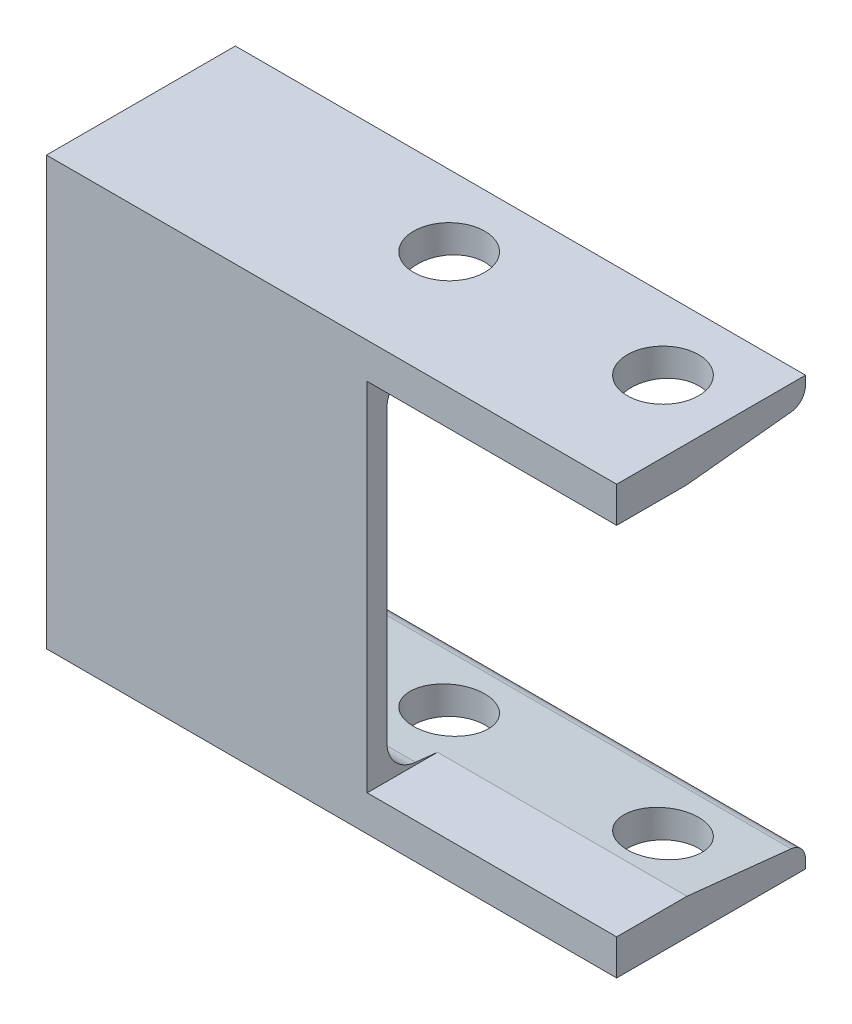
from build123d import *

# Parameters (mm, degrees)
MEMBER_C_12_1_DEPTH = 160
SKETCH_2_W          = 100
SKETCH_2_H          = 100
CUT_EXTRUDE_1_DEPTH = 40
CUT_EXTRUDE_2_REACH = 208.903
SKETCH_3_R          = 10


with BuildPart() as part:
    # Sketch11 → Member C _ 12_1 (new body)
    with BuildSketch(Plane(origin=(0, 0, 0), x_dir=(0, 0, -1), z_dir=(1, 0, 0))):
        with BuildLine():
            Line((53, 120), (0, 120))
            Line((0, 120), (0, 0))
            Line((0, 0), (53, 0))
            Line((53, 0), (53, 2.451956213))
            ThreePointArc((53, 2.451956213), (51.844151715, 5.463043942), (48.970378085, 6.927304742))
            Line((48.970378085, 6.927304742), (13.559243831, 10.649164928))
            ThreePointArc((13.559243831, 10.649164928), (7.811696571, 13.577686529), (5.5, 19.599861986))
            Line((5.5, 19.599861986), (5.5, 100.400138014))
            ThreePointArc((5.5, 100.400138014), (7.811696571, 106.422313471), (13.559243831, 109.350835072))
            Line((13.559243831, 109.350835072), (48.970378085, 113.072695258))
            ThreePointArc((48.970378085, 113.072695258), (51.844151715, 114.536956058), (53, 117.548043787))
            Line((53, 117.548043787), (53, 120))
        make_face()
    extrude(amount=MEMBER_C_12_1_DEPTH)

    # 草图2 → 切除-拉伸1 (cut)
    with BuildSketch(Plane.XY):
        with Locations((140, 60)):
            Rectangle(SKETCH_2_W, SKETCH_2_H)
    extrude(amount=-CUT_EXTRUDE_1_DEPTH, mode=Mode.SUBTRACT)

    # 切除-拉伸2: up to this face of the body (flat: up to its plane)
    cut_extrude_2_end = Plane(part.part.faces().sort_by_distance((80, 120, -26.5))[0])
    # 草图3 → 切除-拉伸2 (cut, up to the picked face)
    with BuildSketch(Plane.XZ, mode=Mode.PRIVATE) as cut_extrude_2_sk1:
        with Locations(Location((140, -33, 0), (0, 0, 270))):
            Circle(SKETCH_3_R)
    cut_extrude_2_tool1 = split(extrude(cut_extrude_2_sk1.sketch, amount=-CUT_EXTRUDE_2_REACH, mode=Mode.PRIVATE), bisect_by=cut_extrude_2_end, keep=Keep.BOTH, mode=Mode.PRIVATE)
    # 草图3 → 切除-拉伸2 (cut, up to the picked face)
    with BuildSketch(Plane.XZ, mode=Mode.PRIVATE) as cut_extrude_2_sk2:
        with Locations(Location((80, -33, 0), (0, 0, 270))):
            Circle(SKETCH_3_R)
    cut_extrude_2_tool2 = split(extrude(cut_extrude_2_sk2.sketch, amount=-CUT_EXTRUDE_2_REACH, mode=Mode.PRIVATE), bisect_by=cut_extrude_2_end, keep=Keep.BOTH, mode=Mode.PRIVATE)
    add(cut_extrude_2_tool1.solids().sort_by(Axis((140, 0, -33), (0, 1, 0)))[0], mode=Mode.SUBTRACT)
    add(cut_extrude_2_tool2.solids().sort_by(Axis((80, 0, -33), (0, 1, 0)))[0], mode=Mode.SUBTRACT)


solid = part.part
